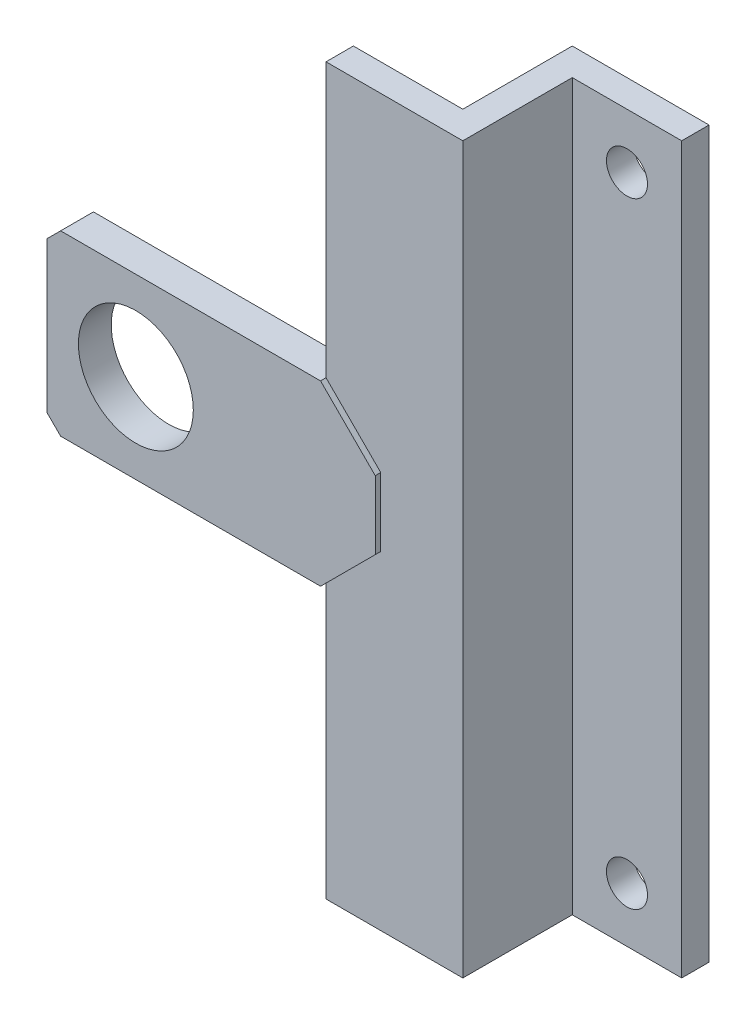
SolidWorks part; units mm, degrees
ref_plane "前视基准面" through (0, 0, 0) normal (0, 0, 1) x (1, 0, 0)
ref_plane "上视基准面" through (0, 0, 0) normal (0, 1, 0) x (1, 0, 0)
ref_plane "右视基准面" through (0, 0, 0) normal (1, 0, 0) x (0, 0, -1)
sketch "草图1" plane through (0, 0, 0) normal (0, 0, 1) x (1, 0, 0)
  line L0 (32.5, 32.5) -> (87.5, 32.5)
  line L1 (-32.5, 32.5) -> (32.5, 32.5)
  line L2 (-32.5, 32.5) -> (-32.5, -32.5)
  line L3 (-32.5, -32.5) -> (32.5, -32.5)
  line L5 (-32.5, 32.5) -> (32.5, -32.5) construction
  line L6 (-32.5, -32.5) -> (32.5, 32.5) construction
  line L7 (87.5, 32.5) -> (87.5, -32.5)
  line L8 (87.5, -32.5) -> (32.5, -32.5)
  circle A0 centre (0, 0) radius 21
  point P0 (0, 0)
  dimension "D3" = 42
  dimension "D1" = 65
  dimension "D2" = 65
  dimension "D4" = 120
extrude "凸台-拉伸1" add sketch "草图1" along normal blind 12
chamfer "倒角1" distance 5 angle 45 2 edges at (-32.5, -32.5, 6) (-32.5, 32.5, 6)
chamfer "倒角2" distance 20 angle 45 2 edges at (87.5, 32.5, 6) (87.5, -32.5, 6)
sketch "草图3" plane through (0, 0, 0) normal (0, 0, -1) x (-1, 0, 0)
  line L0 (-67.5, 32.5) -> (-87.5, 12.5) construction
  line L1 (-87.5, -12.5) -> (-67.5, -32.5) construction
  line L2 (-87.5, -12.5) -> (-87.5, 12.5) construction
  line L3 (-67.5, 32.5) -> (-87.5, 12.5)
  line L4 (-87.5, -12.5) -> (-67.5, -32.5)
  line L5 (-87.5, -12.5) -> (-87.5, 12.5)
  line L6 (-67.5, -32.5) -> (-67.5, -132.5)
  line L7 (-67.5, -132.5) -> (-117.5, -132.5)
  line L8 (-117.5, -132.5) -> (-117.5, 132.5)
  line L9 (-117.5, 132.5) -> (-67.5, 132.5)
  line L10 (-67.5, 132.5) -> (-67.5, 32.5)
  dimension "D1" = 100
  dimension "D2" = 100
  dimension "D3" = 50
extrude "凸台-拉伸2" add sketch "草图3" against normal blind 10
sketch "草图4" plane through (0, 0, 10) normal (0, 0, 1) x (1, 0, 0)
  line L0 (67.5, 132.5) -> (117.5, 132.5) construction
  line L1 (117.5, 132.5) -> (107.5, 132.5)
  line L2 (117.5, 132.5) -> (117.5, -132.5)
  line L3 (117.5, -132.5) -> (107.5, -132.5)
  line L4 (107.5, 132.5) -> (107.5, -132.5)
  line L5 (117.5, -132.5) -> (67.5, -132.5) construction
  line L6 (117.5, 132.5) -> (117.5, -132.5) construction
  dimension "D1" = 10
extrude "凸台-拉伸3" add sketch "草图4" against normal blind 50
sketch "草图6" plane through (0, 0, -40) normal (0, 0, -1) x (-1, 0, 0)
  line L1 (-107.5, -132.5) -> (-157.5, -132.5)
  line L2 (-107.5, -132.5) -> (-107.5, 132.5)
  line L3 (-107.5, 132.5) -> (-157.5, 132.5)
  line L4 (-157.5, -132.5) -> (-157.5, 132.5)
  point P5 (-107.5, 132.5)
  dimension "D1" = 50
extrude "凸台-拉伸4" add sketch "草图6" against normal blind 10
sketch "草图7" plane through (0, 0, -30) normal (0, 0, 1) x (1, 0, 0)
  line L0 (137.5, 132.5) -> (137.5, -132.5) construction
  line L1 (117.5, 132.5) -> (157.5, 132.5) construction
  line L2 (157.5, -132.5) -> (117.5, -132.5) construction
  circle A0 centre (137.5, 112.5) radius 7.5
  circle A1 centre (137.5, -112.5) radius 7.5
  dimension "D1" = 15
  dimension "D2" = 20
  dimension "D3" = 20
  dimension "D4" = 15
extrude "切除-拉伸1" cut sketch "草图7" against normal through all
